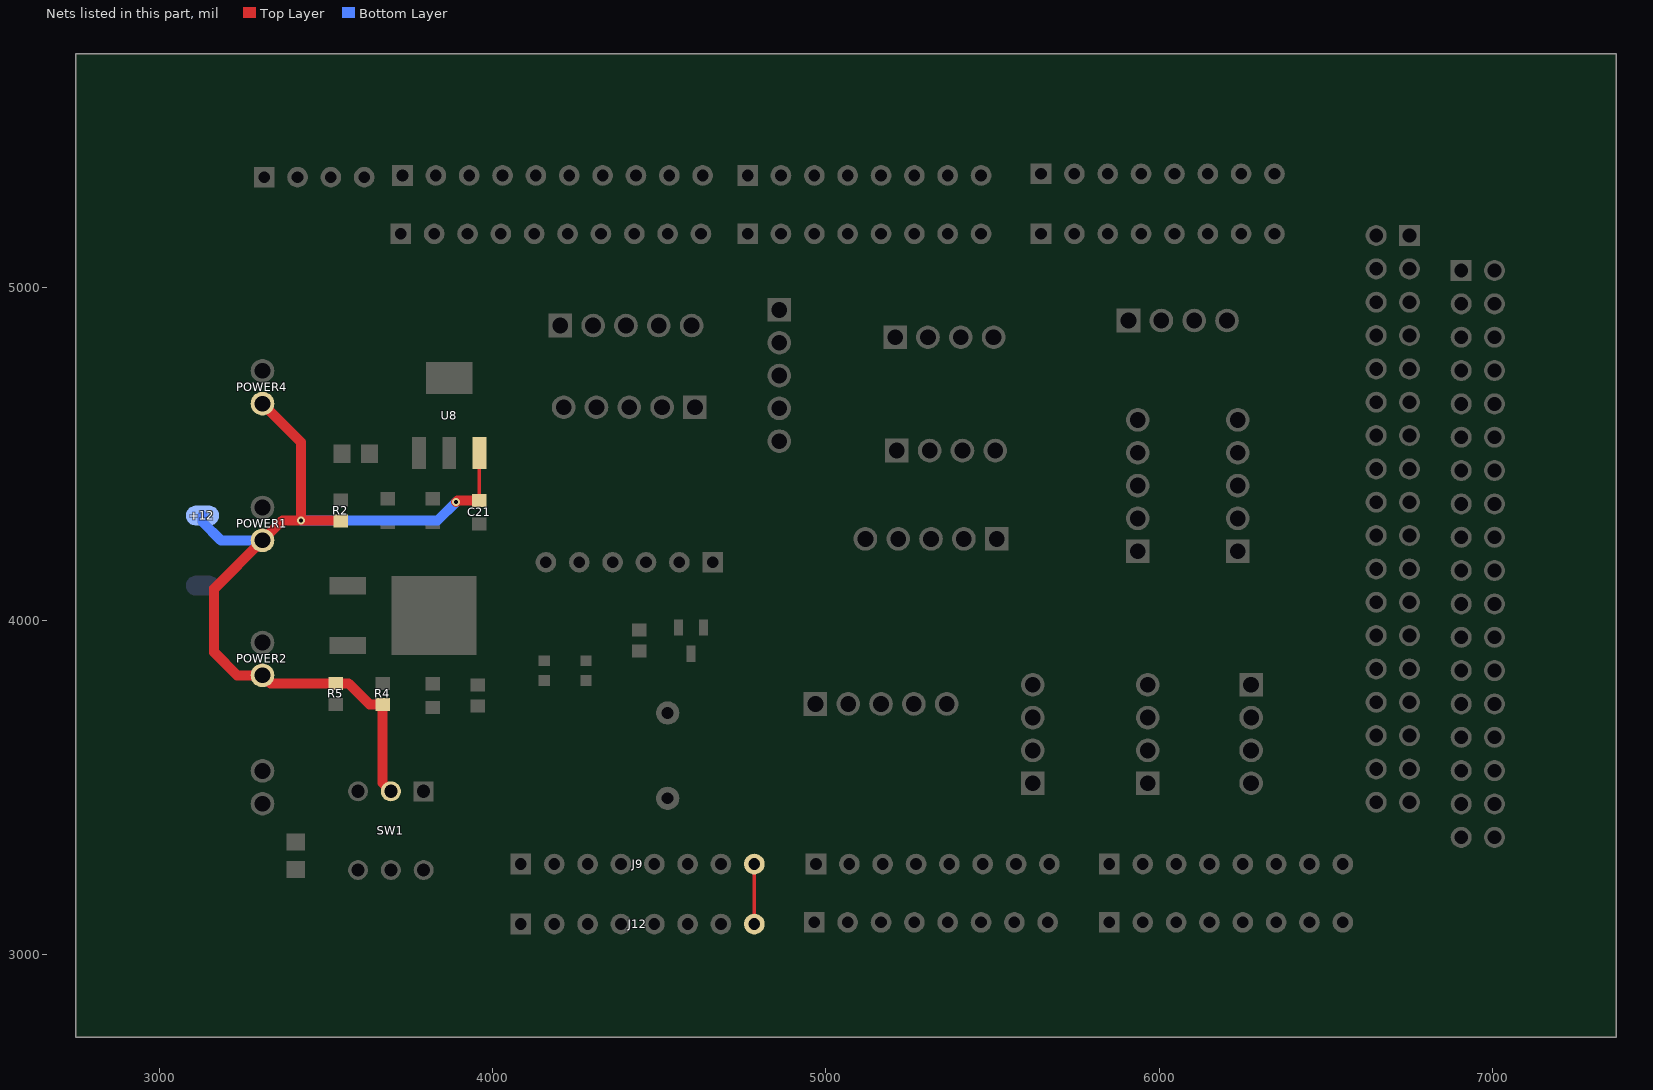
[diagram p0: the nets of this part, all layers, seen from the top]
# Altium PCB MISC49934.pcbdoc (part 2 of 2)
Units mil, origin at the board's own origin, x right, y up, seen from the top; angles counter-clockwise.
Board outline 4620 x 2950 mil, 2 copper layers (Top Layer, Bottom Layer), stack 0 mil thick; 53 components, 145 nets, 295 pads, 118 vias.

## Via types
v1: diameter 24, hole 12, Top Layer to Bottom Layer, 118 vias

## Nets (pads, with @x,y where several pads share a name; then routed paths per layer and width w, separated by ;. In a path a pad name is that pad's centre, name@x,y a point inside that pad or via, vN(x,y) a via of type N, cw(c..) or ccw(c..) an arc to the next point about the centre after c; other vN are vias at no path point) (continued)
VCC: +12.1 C21.2 POWER1.1 POWER2.1 POWER4.1 R2.2 R4.1 R5.1 SW1.2 U8.3 | length 2824.3
  Top Layer w10: C21.2@3960,4360.44 3960,4502 U8.3@3960.55,4502.5
  Top Layer w30: POWER2.1@3310,3835.7 3334.3,3811.5 R5.1@3530,3811.49 3568.5,3811.5 3631.5,3748.5 R4.1@3670,3748.51 3670,3513.1 SW1.2@3695.01,3488.11 ; POWER2.1@3310,3835.75 3234.25,3835.75 3165,3905 3165,4095.75 POWER1.1@3310,4240.75 3369.25,4300 v1(3425,4300) ; POWER4.1@3310,4650.7 3425,4535.7 v1(3425,4300) ; v1@3420,4300 v1(3425,4300) ; R2.2@3545,4298.5 3543.5,4300 v1(3425,4300) ; v1(3890,4355) 3895.4,4360.4 C21.2@3960,4360.44
  Bottom Layer w30: +12.1@3130,4315 3130,4295.7 3185,4240.7 POWER1.1@3310,4240.7 ; v1(3425,4300) 3835,4300 v1(3890,4355)
VIN: J9.8 J12.8 | length 180
  Top Layer w10: J12.8@4785,3090 J9.8@4785,3270
pads on no net: HC-06.1 HC-06.6 J9.1 J12.1 SW1.1 SW1.4 SW1.5 SW1.6 U8.4

## Polygon pours and split planes (outlines as drawn)
GND on Bottom Layer (solid, remove dead copper, pour order 4): 3005,5450 3000,5445 3000,3005 7110,3005 7110,5430
GND on Top Layer (solid, remove dead copper, pour order 4): 3000,5390 3005,5385 3005,3005 3010,3000 7120,3000 7105,3015 7105,5385

## Keep-outs
Board Outline Layer:
  lines w10: 3005.87,3173.07 ccw(c3025.55,3173.07) 3025.55,3153.39
  lines w10 net S$14301: 3005.87,3173.07 3005.87,5220.31 3006,5333 ; 3006,5324.53 cw(c3060,5330.87) 3065,5385
  lines w10 net S$3075: 6830.15,5240 6975,5240 7110,5105 7110,3285 6978.39,3153.39 6844.45,3153.39
  lines w10 net S$3947: 3890.47,3151 3907.3,3132.7 4030,3010 6610,3010 6705,3125 6729.9,3153.4
  lines w10 net S$3949: 3564,5385 3596,5385 3665,5385 6395,5385
  lines w10 net S$3952: 3055,5385 3519.55,5385
  lines w10 net S$3954: 6539.9,5240 6830.15,5240
  lines w10 net S$3958: 3025.55,3153.39 3887.66,3153.39
  lines w10 net S$3961: 3887.66,3153.39 3907.3,3133.75 3907.3,3132.7
  lines w10 net S$3963: 6705,3125 6729.9,3153.4
  lines w10 net S$3965: 6729.9,3153.39 6844.45,3153.39
  lines w10 net S$3975: 6395,5385 6539.9,5240
  lines w10 net S$3977: 3519.55,5385 3665,5385

## Other copper
Top Layer:
  drawing of 345 lines, arcs and shapes, not listed
Bottom Layer:
  region net OUT1_+5V: 3882.94,4411 3882.94,4429 3891.34,4425 3891.34,4415
  region net OUT1_+5V: 4172.06,4521 4172.06,4539 4163.66,4535 4163.66,4525
  region net VCC: 3150,4285 3110,4285 3163.79,4240.75 3195.61,4251.36
  region net VCC: 3286.56,4214.17 3286.56,4267.32 3261.76,4255.75 3261.76,4225.75
  region net +5V_3: 4697.94,4381 4697.94,4399 4706.34,4395 4706.34,4385
  region net +5V_3: 4902.06,4381 4902.06,4399 4893.66,4395 4893.66,4385
  region net D37: 6718.57,4353.03 6751.97,4386.43 6723.21,4388.86 6716.14,4381.79
  region net D37: 6326.98,4029.25 6314.25,4041.98 6323.02,4045.09 6330.09,4038.02
  region net D52: 6873.57,3448.03 6906.97,3481.43 6878.21,3483.86 6871.14,3476.79
  region net D52: 6679.02,3567.23 6658.51,3524.67 6686.32,3531.61 6690.92,3541.15
  region net D52: 6629.17,3531.38 6629.17,3578.62 6607.12,3560 6607.12,3550
  region net D52: 6556,3502.94 6574,3502.94 6570,3511.34 6560,3511.34
  region net D48: 5691.79,3347.26 5680.77,3333.02 5689.05,3330 5696.79,3340
  region net D48: 6646.76,3723.67 6619.32,3762.13 6612.15,3734.22 6618.04,3725.97
  region net D46: 6551,3952.06 6569,3952.06 6565,3945 6555,3945
  region net D46: 6618.57,3853.03 6651.97,3886.43 6623.21,3888.86 6616.14,3881.79
  region net D47: 6516,3977.06 6534,3977.06 6530,3968.66 6520,3968.66
  region net D47: 6536.14,3885.31 6519,3879.8 6520,3888.95 6530,3892.16
  region net D42: 6873.57,3948.03 6906.97,3981.43 6878.21,3983.86 6871.14,3976.79
  region net D42: 6679.02,4067.23 6658.51,4024.67 6686.32,4031.61 6690.92,4041.15
  region net D42: 6618.57,4056.97 6651.97,4023.57 6623.21,4021.14 6616.14,4028.21
  region net D42: 5261.19,3714.64 5298.79,3752.2 5301.06,3719.41 5293.99,3712.34
  region net D43: 5359.6,3714.64 5397.22,3752.19 5398.54,3720.33 5391.46,3713.27
  region net D43: 6718.57,4053.03 6751.97,4086.43 6723.21,4088.86 6716.14,4081.79
  region net D40: 6629.17,4131.38 6629.17,4178.62 6610,4160 6610,4150
  region net D40: 6541.98,4074.25 6529.25,4086.98 6538.02,4090.09 6545.09,4083.02
  region net D41: 6973.57,4048.03 7006.97,4081.43 6978.21,4083.86 6971.14,4076.79
  region net D41: 6770.83,4131.38 6770.83,4178.62 6792.88,4160 6792.88,4150
  region net D41: 6718.57,4153.03 6751.97,4186.43 6723.21,4188.86 6716.14,4181.79
  region net D41: 6541.98,4109.25 6529.25,4121.98 6538.02,4125.09 6545.09,4118.02
  region net D19: 6436,4957.94 6454,4957.94 6450,4966.34 6440,4966.34
  region net D19: 6174.8,5168.54 6132.8,5188.5 6158.32,5200.4 6167.91,5195.84
  region net D19: 6235.75,4733.02 6223.02,4745.75 6219.91,4736.98 6226.98,4729.91
  region net D39: 6973.57,4148.03 7006.97,4181.43 6978.21,4183.86 6971.14,4176.79
  region net D39: 6770.83,4231.38 6770.83,4278.62 6792.88,4260 6792.88,4250
  region net D39: 6744.14,4285.95 6720.03,4245.31 6710.49,4272.44 6715.75,4281.32
  region net D36: 6884.17,4226.38 6884.17,4273.62 6865,4255 6865,4245
  region net D36: 6679.02,4367.23 6658.51,4324.67 6686.32,4331.61 6690.92,4341.15
  region net D37: 6973.57,4248.03 7006.97,4281.43 6978.21,4283.86 6971.14,4276.79
  region net D37: 6770.83,4331.38 6770.83,4378.62 6792.88,4360 6792.88,4350
  region net D36: 6366.98,4029.25 6354.25,4041.98 6363.02,4045.09 6370.09,4038.02
  region net D28: 6873.57,4648.03 6906.97,4681.43 6878.21,4683.86 6871.14,4676.79
  region net D28: 6677.83,4769.76 6661.16,4725.55 6688.19,4734.74 6692.06,4745.01
  region net D35: 6748.03,4486.43 6781.43,4453.03 6783.86,4481.79 6776.79,4488.86
  region net D34: 6491.98,4334.25 6479.25,4346.98 6488.02,4350.09 6495.09,4343.02
  region net D34: 6629.17,4431.38 6629.17,4478.62 6607.12,4460 6607.12,4450
  region net D26: 6873.57,4748.03 6906.97,4781.43 6878.21,4783.86 6871.14,4776.79
  region net D26: 6648.03,4823.57 6681.43,4856.97 6683.86,4828.21 6676.79,4821.14
  region net D24: 6873.57,4848.03 6906.97,4881.43 6878.21,4883.86 6871.14,4876.79
  region net D24: 6648.03,4923.57 6681.43,4956.97 6683.86,4928.21 6676.79,4921.14
  region net D25: 6973.57,4848.03 7006.97,4881.43 6978.21,4883.86 6971.14,4876.79
  region net D25: 6770.83,4931.38 6770.83,4978.62 6792.88,4960 6792.88,4950
  region net D23: 6973.57,4948.03 7006.97,4981.43 6978.21,4983.86 6971.14,4976.79
  region net D23: 6770.83,5031.38 6770.83,5078.62 6792.88,5060 6792.88,5050
  region net D24: 6485.75,4838.02 6473.02,4850.75 6469.91,4841.98 6476.98,4834.91
  region net D24: 6391,4722.94 6409,4722.94 6405,4731.34 6395,4731.34
  region net +5V_1: 4183.06,3300.94 4215.94,3268.06 4218.38,3296.31 4211.31,3303.38
  region net +5V_1: 4501.85,3440.75 4501.85,3493.25 4477.35,3472 4477.35,3462
  region net D30: 6530.75,4143.02 6518.02,4155.75 6514.91,4146.98 6521.98,4139.91
  region net D30: 5500.31,3426.14 5494.8,3409 5503.95,3410 5507.16,3420
  region net D15: 4692.94,4346 4692.94,4364 4701.34,4360 4701.34,4350
  region net D51: 5816.98,3960.75 5804.25,3948.02 5811.46,3946.46 5818.54,3953.54
  region net D52: 5763.86,4019.69 5781,4025.2 5780,4016.05 5770,4012.84
  region net D52: 5766,3892.94 5784,3892.94 5780,3901.34 5770,3901.34
  region net D50: 5676.98,4075.75 5664.25,4063.02 5673.02,4059.91 5680.09,4066.98
  region net D50: 5726,3892.94 5744,3892.94 5740,3901.34 5730,3901.34
  region net D40: 5556.98,4094.25 5544.25,4106.98 5553.02,4110.09 5560.09,4103.02
  region net D41: 5547.94,4141 5547.94,4159 5556.34,4155 5556.34,4145
  region net +5V_4: 5462.94,4726 5462.94,4744 5471.34,4740 5471.34,4730
  region net +5V_4: 5585.75,4798.02 5573.02,4810.75 5569.91,4801.98 5576.98,4794.91
  region net D20: 5332.94,4701 5332.94,4719 5341.34,4715 5341.34,4705
  region net D20: 5600.49,4773.88 5594.53,4790.86 5587.75,4784.82 5591.42,4774.35
  region net D20: 6268.25,5139.5 6221.75,5139.5 6240,5117.8 6250,5117.8
  region net D20: 6196.98,4999.25 6184.25,5011.98 6193.02,5015.09 6200.09,5008.02
  region net D18: 6130.78,4923.44 6077.63,4923.44 6099.21,4948.24 6109.21,4948.24
  region net D18: 6043.06,5129.06 6075.94,5161.94 6078.38,5133.69 6071.31,5126.62
  region net D11: 4276.21,4637.78 4313.79,4675.36 4281,4677.65 4273.93,4670.57
  region net D1: 4309.73,5017.97 4291.81,5016.23 4296.58,5008.25 4306.58,5009.23
  region net D1: 4328.15,4908.43 4275,4908.44 4296.58,4933.24 4306.58,4933.24
  region net D11: 4339.72,5132.72 4296.09,5148.8 4305.23,5122.31 4315.57,5118.5
  region net D11: 4266.98,5064.25 4254.25,5076.98 4263.02,5080.09 4270.09,5073.02
  region net D8: 4116.14,4779.69 4099,4785.2 4100,4776.05 4110,4772.84
  region net D8: 4096,4707.94 4114,4707.94 4110,4716.34 4100,4716.34
  region net D15: 5001,4822.94 5019,4822.94 5015,4831.34 5005,4831.34
  region net D15: 5001,4887.06 5019,4887.06 5015,4878.66 5005,4878.66
  region net D49: 5831.98,4040.75 5819.25,4028.02 5828.02,4024.91 5835.09,4031.98
  region net D31: 6516,3697.94 6534,3697.94 6530,3706.34 6520,3706.34
  region net OUT1_+5V: 5080.75,4076.56 5068.02,4089.28 5064.91,4080.52 5071.98,4073.45
  region net OUT1_+5V: 4981.95,3976.09 4967.43,3986.72 4975.57,3991.17 4983.73,3985.19
  region net D7: 5885.75,3656.98 5873.02,3644.25 5869.91,3653.02 5876.98,3660.09
  region net D24: 6046,4562.94 6064,4562.94 6060,4571.34 6050,4571.34
  region net D24: 6046,4562.94 6064,4562.94 6060,4571.34 6050,4571.34
  region net D10: 4681,4992.06 4699,4992.06 4695,4983.66 4685,4983.66
  region net D10: 4824.64,4732.78 4862.22,4770.36 4829.42,4772.65 4822.35,4765.58
  region net D51: 5566,3967.94 5584,3967.94 5580,3976.34 5570,3976.34
  region net D51: 5563.86,4059.69 5581,4065.2 5580,4056.05 5570,4052.84
  region net D7: 5531.98,3980.75 5519.25,3968.02 5528.02,3964.91 5535.09,3971.98
  region net D7: 5697.06,3816 5697.06,3834 5688.66,3830 5688.66,3820
  region net D21: 5277.94,5016 5277.94,5034 5286.34,5030 5286.34,5020
  region net D15: 5410.75,4993.02 5398.02,5005.75 5396.46,4998.54 5403.54,4991.46
  region net D15: 5277.94,4986 5277.94,5004 5286.34,5000 5286.34,4990
  region net D14: 5527.06,5016 5527.06,5034 5518.66,5030 5518.66,5020
  region net D14: 5232.94,4956 5232.94,4974 5241.34,4970 5241.34,4960
  region net OUT1_+5V: 4824.64,4535.93 4862.22,4573.52 4829.43,4575.8 4822.35,4568.73
  region net OUT1_+5V: 4700.15,4571 4700.15,4589 4708.55,4585 4708.55,4575
  region net D7: 4770.75,5088.02 4758.02,5100.75 4754.91,5091.98 4761.98,5084.91
  region net D7: 4721,5007.94 4739,5007.94 4735,5016.34 4725,5016.34
  region net D39: 4407.78,4604.64 4445.36,4642.22 4447.65,4609.42 4440.58,4602.35
  region net OUT1_+5V: 5091.98,4087.78 5079.25,4100.51 5088.02,4103.62 5095.09,4096.55
  region net OUT1_+5V: 5144.72,4221.56 5091.57,4221.56 5113.15,4196.76 5123.15,4196.76
  region net D14: 5086,4837.94 5104,4837.94 5100,4846.34 5090,4846.34
  region net D14: 5086,4927.06 5104,4927.06 5100,4918.66 5090,4918.66
  region net D14: 5086,4927.06 5104,4927.06 5100,4918.66 5090,4918.66
  region net D20: 4831.53,4171.67 4821.86,4186.86 4831.03,4188.1 4836.53,4179.46
  region net D20: 4955.75,4293.02 4943.02,4305.75 4939.91,4296.98 4946.98,4289.91
  region net D14: 4935.75,4323.02 4923.02,4335.75 4919.91,4326.98 4926.98,4319.91
  region net D14: 4777.94,4201 4777.94,4219 4786.34,4215 4786.34,4205
  region net D48: 5060.75,4183.02 5048.02,4195.75 5044.91,4186.98 5051.98,4179.91
  region net D48: 4911.67,4056.53 4926.86,4046.86 4928.1,4056.03 4919.46,4061.53
  region net D2: 4966,4272.06 4984,4272.06 4980,4263.66 4970,4263.66
  region net D2: 4846.98,4114.25 4834.25,4126.98 4843.02,4130.09 4850.09,4123.02
  region net D31: 5655.16,3803.27 5611.26,3773.31 5642.99,3764.94 5651.4,3770.67
  region net D31: 5830.75,3596.98 5818.02,3584.25 5814.91,3593.02 5821.98,3600.09
  region net D31: 5840.31,3591.14 5834.8,3574 5843.95,3575 5847.16,3585
  region net D48: 4874.94,3397.01 4857.07,3394.85 4860,3403.67 4870,3404.87
  region net D48: 4856,3547.06 4874,3547.06 4870,3538.66 4860,3538.66
  region net D38: 5885.2,3486 5879.69,3468.86 5872.84,3475 5876.05,3485
  region net D38: 5461.98,3545.75 5449.25,3533.02 5458.02,3529.91 5465.09,3536.98
  region net D38: 4777.94,3586 4777.94,3604 4786.34,3600 4786.34,3590
  region net D38: 4907.06,3586 4907.06,3604 4898.66,3600 4898.66,3590
  region net OUT1_+5V: 5915.57,4572.22 5908.03,4624.83 5886.53,4600 5887.97,4590
  region net OUT1_+5V: 5667.06,4356 5667.06,4374 5658.66,4370 5658.66,4360
  region net OUT1_+5V: 5496.98,4380.75 5484.25,4368.02 5493.02,4364.91 5500.09,4371.98
  region net OUT1_+5V: 5496.98,4380.75 5484.25,4368.02 5493.02,4364.91 5500.09,4371.98
  region net D31: 6411,3872.94 6429,3872.94 6425,3881.34 6415,3881.34
  region net D31: 6510.75,4173.02 6498.02,4185.75 6494.91,4176.98 6501.98,4169.91
  region net D38: 6386,4022.06 6404,4022.06 6400,4013.66 6390,4013.66
  region net D38: 6386,3827.94 6404,3827.94 6400,3836.34 6390,3836.34
  region net D36: 6366.98,4030.75 6354.25,4018.02 6363.02,4014.91 6370.09,4021.98
  region net D36: 6361,3887.94 6379,3887.94 6375,3896.34 6365,3896.34
  region net D37: 6272.78,3547.71 6310.36,3510.13 6312.65,3542.93 6305.58,3550
  region net D37: 6306,4022.06 6324,4022.06 6320,4013.66 6310,4013.66
  region net D19: 6239.64,3608.57 6277.22,3646.15 6244.42,3648.44 6237.35,3641.37
  region net D19: 6174.8,5168.54 6132.8,5188.5 6158.32,5200.4 6167.91,5195.84
  region net D15: 5696,5067.94 5714,5067.94 5710,5076.34 5700,5076.34
  region net D15: 5714.06,5161.94 5746.94,5129.06 5718.69,5126.62 5711.62,5133.69
  region net D14: 5506,5107.06 5524,5107.06 5520,5098.66 5510,5098.66
  region net D14: 5535.75,5036.98 5523.02,5024.25 5519.91,5033.02 5526.98,5040.09
  region net +5V_3: 5332.37,4873.44 5279.22,4873.44 5300.79,4895.79 5310.79,4895.79
  region net +5V_3: 5702.06,4966 5702.06,4984 5693.66,4980 5693.66,4970
  region net D5: 4963.06,5190.94 4995.94,5158.06 4998.38,5186.31 4991.31,5193.38
  region net D5: 5894.85,4935.43 5919.85,4935.43 5912.35,4937.65 5902.35,4937.65
  region net D3: 5163.06,5190.94 5195.94,5158.06 5198.38,5186.31 5191.31,5193.38
  region net D3: 5988.44,3682.63 5988.44,3735.78 6013.24,3714.21 6013.24,3704.21
  region net D33: 5962.78,3843.01 6000.36,3805.43 6002.65,3838.22 5995.58,3845.3
  region net D6: 6262.5,3843.08 6287.5,3843.08 6280,3858.08 6270,3858.08
  region net D6: 6266,3952.06 6284,3952.06 6280,3943.66 6270,3943.66
  region net D2: 5265.75,5093.02 5253.02,5105.75 5249.91,5096.98 5256.98,5089.91
  region net D2: 5057.94,5016 5057.94,5034 5066.34,5030 5066.34,5020
  region net D2: 5041,5017.06 5059,5017.06 5055,5008.66 5045,5008.66
  region net D2: 5041,4682.94 5059,4682.94 5055,4691.34 5045,4691.34
  region net D6: 4863.06,5129.06 4895.94,5161.94 4898.38,5133.69 4891.31,5126.62
  region net D6: 5961,3967.94 5979,3967.94 5975,3976.34 5965,3976.34
  region net D33: 6565.75,4498.02 6553.02,4510.75 6549.91,4501.98 6556.98,4494.91
  region net D33: 6231.98,4034.25 6219.25,4046.98 6228.02,4050.09 6235.09,4043.02
  region net D34: 6003.57,4864.64 6041.15,4902.22 6043.44,4869.42 6036.37,4862.35
  region net D32: 6181,3882.94 6199,3882.94 6195,3891.34 6185,3891.34
  region net D32: 6560.75,4453.02 6548.02,4465.75 6544.91,4456.98 6551.98,4449.91
  region net D34: 6003.57,4864.64 6041.15,4902.22 6043.44,4869.42 6036.37,4862.35
  region net D34: 6351,4387.94 6369,4387.94 6365,4396.34 6355,4396.34
  region net D8: 4805.75,4071.98 4793.02,4059.25 4789.91,4068.02 4796.98,4075.09
  region net D8: 4377.94,4486 4377.94,4504 4386.34,4500 4386.34,4490
  region net D10: 4453.91,5171.2 4410.28,5187.28 4434.43,5201.5 4444.77,5197.69
  region net D10: 4681,5112.94 4699,5112.94 4695,5121.34 4685,5121.34
  region net D10: 4681,5097.06 4699,5097.06 4695,5088.66 4685,5088.66
  region net D10: 4681,5007.94 4699,5007.94 4695,5016.34 4685,5016.34
  region net Q2_3: 3336.57,3572.69 3283.43,3572.69 3305,3597.49 3315,3597.49
  region net _SDA: 3613.06,5299.06 3645.94,5331.94 3648.38,5303.69 3641.31,5296.62
  region net _SDA: 3844.72,5307.72 3801.09,5323.8 3810.23,5297.31 3820.57,5293.5

## Silkscreen, mask and mechanical layers (free items; w line width, h text height)
Top Silkscreen Layer:
  lines w10 net S$11567: 3355.56,5195 3355.56,5280 ; 3465.56,5195 3465.56,5280 ; 3660,5192.5 3660,5277.5 ; 4235,4410 4235,4502.2 ; 4295,4225 4295,4315 ; 4339.28,4410 4339.28,4502.2 ; 4405,4225 4405,4320 ; 4453,4502.2 4453.28,4410 ; 4504,4225 4505,4325 ; 4559,4502.2 4560,4410 ; 4605,4320 4605.5,4225 ; 4665,4410 4665,4502.2 ; 5005,3565 5005,3659.45 ; 5109.01,3659.45 5110,3570 ; 5200,3570 5201.01,3659.45 ; 5298.01,3574.45 5298.01,3659.45 ; 5405.01,3574.45 5405.01,3659.45 ; 5715,3680 5800,3680 ; 5716,3482.39 5801,3482.39 ; 5716,3574.39 5801,3574.39 ; 5716,3784.39 5801,3784.39 ; 6061,3476.97 6146,3476.97 ; 6061,3579.36 6146,3579.36 ; 6061,3673.86 6146,3673.86 ; 6061,3778.91 6146,3778.91 ; 6408,3484.74 6493,3484.74 ; 6408,3585.46 6493,3585.46 ; 6408,3695.75 6493,3695.75 ; 6408,3786.86 6493,3786.86
  lines w10 net S$11623: 3560,5190 3560,5277.44 3562.56,5280
  lines w10 net S$12201: 5345,4650 5345,4720
  lines w10 net S$12203: 5445,4650 5445,4720
  lines w10 net S$12205: 5558.54,4643 5558.54,4715
  lines w10 net S$12209: 5230.82,4643 5230.82,4720
  lines w10 net S$12241: 5225.7,4983 5225.7,5050
  lines w10 net S$12243: 5329.7,4983 5329.7,5050
  lines w10 net S$12245: 5433.7,4983 5433.7,5055
  lines w10 net S$12247: 5539.7,4983 5539.7,5055
  lines w10 net S$12361: 6325,4176.58 6410,4176.58
  lines w10 net S$12363: 6325.55,4277.78 6390,4277.78
  lines w10 net S$12365: 6325.55,4393.78 6400,4393.78
  lines w10 net S$12369: 6325,4586.78 6405,4586.78
  lines w10 net S$12371: 6325.55,4490.28 6405,4490.28
  lines w10 net S$12373: 5932.39,4745 5932.39,4804
  lines w10 net S$12375: 6034.39,4804 6035,4745
  lines w10 net S$12377: 6135.39,4740 6135.39,4804
  lines w10 net S$12379: 6245,4740 6245,4804
  lines w10 net S$12417: 4997.8,4914.7 5080,4914.7
  lines w10 net S$12419: 4997.8,4798.27 5080,4798.27
  lines w10 net S$12421: 4997.8,4720.41 5080,4720.41
  lines w10 net S$12423: 4997.8,4607.56 5080,4607.56
  lines w10 net S$12425: 4997.8,4501.41 5065,4501.41
  lines w10 net S$12427: 5065,4501.41 5080,4501.41
  lines w10 net S$12429: 4231.58,4745 4231.58,4795
  lines w10 net S$12431: 4336.27,4745 4336.27,4794.45
  lines w10 net S$12433: 4454.41,4745 4454.41,4794.45
  lines w10 net S$12435: 4570,4745 4570,4795
  lines w10 net S$12437: 4682.53,4745 4682.53,4794.45
  lines w10 net S$12583: 5155.87,4015 5155.87,4107.2
  lines w10 net S$12586: 5262.53,4015 5262.53,4107.2
  lines w10 net S$12588: 5355.37,4015 5355.37,4107.2
  lines w10 net S$12590: 5458.87,4015 5458.87,4107.2
  lines w10 net S$12592: 5580.87,4015 5580.87,4107.2
  lines w10 net S$12594: 5710,4572.15 5797.2,4572.15
  lines w10 net S$12596: 5705,4464.15 5797.2,4464.15
  lines w10 net S$12598: 5705,4348.15 5797.2,4348.15
  lines w10 net S$12601: 5700,4268.15 5797.2,4268.15
  lines w10 net S$12603: 5700,4155.81 5797.2,4155.81
  lines w10 net S$14520: 3330,4850 3405,4775 3405,4360
  lines w10 net S$3942: 3310,3740 3330,3740 3405,3815 3405,4360
  text "D6" at 4855,5240 h39.37
  text "D15" at 5730,5240 h39.37
  text "D21" at 6330,5239.6 h39.37
  text "AREF" at 3895,5235 h39.37
  text "GND" at 4010,5235 h39.37
  text "D12" at 4205,5235 h39.37
  text "D11" at 4310,5235 h39.37
  text "D10" at 4410,5235 h39.37
  text "D9" at 4510,5235 h39.37
  text "D8" at 4615,5235 h39.37
  text "D7" at 4750,5234.6 h39.37
  text "D5" at 4950,5235 h39.37
  text "D4" at 5050,5234.6 h39.37
  text "D3" at 5160,5235 h39.37
  text "D2" at 5250,5234.6 h39.37
  text "D1" at 5355,5234.6 h39.37
  text "D0" at 5450,5235 h39.37
  text "D14" at 5625,5234.6 h39.37
  text "D16" at 5825,5235 h39.37
  text "D17" at 5920,5234.6 h39.37
  text "D18" at 6030,5235 h39.37
  text "D19" at 6130,5235.2 h39.37
  text "D20" at 6230,5235 h39.37
  text "SCL" at 3700,5230 h39.37
  text "SDA" at 3805,5230 h39.37
  text "D13" at 4105,5230 h39.37
  text "SCL" at 3440,5185 h59.05 r90
  text "+5V" at 3535,5185 h59.05 r90
  text "SDA" at 3340,5170 h59.05 r90
  text "GND" at 3635,5165 h59.05 r90
  text "5V" at 6540,5145 h39.37
  text "5V" at 6810,5145 h39.37
  text "D23" at 6810,5110 h39.37 r270
  text "TX" at 5670,5065 h59.05 r90
  text "TX" at 5870,5065 h59.05 r90
  text "RX" at 5770,5060 h59.05 r90
  text "RX" at 5965,5055 h59.05 r90
  text "Servo signal line" at 4370,5050 h59.05
  text "RX" at 6070,5050 h59.05 r90
  text "TX" at 6165,5050 h59.05 r90
  text "D22" at 6535,5035 h39.37
  text "SDA" at 6265,5030 h59.05 r90
  text "SCL" at 6370,5030 h59.05 r90
  text "V0.2" at 3255,4995 h59.05
  text "GND" at 5220,4990 h43.31 r90
  text "D49" at 5420,4990 h43.31 r90
  text "D50" at 5525,4990 h43.31 r90
  text "+5V" at 5325,4985 h43.31 r90
  text "D25" at 6815,4985 h39.37 r270
  text "D24" at 6535,4945 h39.37
  text "GND" at 5010,4925 h43.31
  text "D26" at 6815,4885 h39.37 r270
  text "D26" at 6540,4835 h39.37
  text "OUT" at 5015,4820 h43.31
  text "PWC" at 5890,4795 h43.31 r270
  text "IN3" at 5975,4795 h43.31 r270
  text "A3" at 6080,4790 h43.31 r270
  text "B3" at 6180,4790 h43.31 r270
  text "D29" at 6815,4770 h39.37 r270
  text "Output" at 3060,4745 h78.74
  text "S3" at 4370,4745 h59.05
  text "S4" at 4490,4745 h59.05
  text "S5" at 4600,4745 h59.05
  text "S1" at 4160,4740 h59.05
  text "S2" at 4255,4740 h59.05
  text "D29" at 6535,4735 h39.37
  text "S2" at 5015,4730 h43.31
  text "D31" at 6815,4680 h39.37 r270
  text "+5V" at 5330,4660 h59.05 r90
  text "D51" at 5425,4655 h59.05 r90
  text "GND" at 5225,4650 h43.31 r90
  text "D52" at 5545,4650 h59.05 r90
  text "D30" at 6540,4635 h39.37
  text "Power" at 3060,4630 h78.74
  text "S3" at 5020,4625 h43.31
  text "+5V" at 5720,4595 h43.31
  text "+5V" at 6330,4590 h43.31
  text "D33" at 6815,4580 h39.37 r270
  text "D32" at 6540,4540 h39.37
  text "+5V" at 5005,4505 h43.31
  text "L" at 6355,4500 h43.31
  text "L" at 5735,4490 h43.31
  text "D35" at 6810,4475 h39.37 r270
  text "S1" at 4165,4435 h59.05
  text "LED" at 4350,4435 h59.05
  text "S0" at 4260,4430 h59.05
  text "D34" at 6535,4430 h39.37
  text "C" at 6345,4410 h43.31
  text "+5V" at 4630,4400 h59.05 r90
  text "C" at 5735,4395 h43.31
  text "GND" at 4530,4385 h59.05 r90
  text "D37" at 6810,4385 h39.37 r270
  text "D36" at 6535,4345 h39.37
  text "Servo" at 3050,4330 h78.74
  text "R" at 6350,4290 h43.31
  text "R" at 5740,4280 h43.31
  text "D39" at 6815,4280 h39.37 r270
  text "Bluetooth" at 4075,4260 h59.05
  text "RX" at 4480,4250 h59.05 r90
  text "TX" at 4580,4250 h59.05 r90
  text "D38" at 6540,4240 h39.37
  text "+5V" at 4280,4235 h59.05 r90
  text "GND" at 4380,4235 h59.05 r90
  text "Power" at 3045,4230 h78.74
  text "GND" at 6330,4190 h43.31
  text "GND" at 5700,4185 h43.31
  text "D41" at 6815,4175 h39.37 r270
  text "D40" at 6540,4145 h39.37
  text "+5V" at 5090,4100 h59.05 r270
  text "GND" at 5490,4100 h59.05 r270
  text "LED" at 5195,4090 h59.05 r270
  text "D43" at 6820,4075 h39.37 r270
  text "D42" at 6535,4045 h39.37
  text "S0" at 5290,4035 h59.05
  text "S1" at 5385,4035 h59.05
  text "D45" at 6820,3980 h39.37 r270
  text "D44" at 6535,3920 h39.37
  text "Motor" at 3045,3915 h78.74
  text "OUT-12V" at 3485,3895 h59.05 r90
  text "D47" at 6815,3885 h39.37 r270
  text "D46" at 6535,3835 h39.37
  text "Power" at 3045,3825 h78.74
  text "B2" at 6070,3795 h59.05
  text "PWD" at 6420,3795 h59.05
  text "B1" at 5725,3790 h59.05
  text "D49" at 6815,3775 h39.37 r270
  text "D48" at 6535,3740 h39.37
  text "IN4" at 6420,3700 h59.05
  text "A2" at 6065,3695 h59.05
  text "A1" at 5725,3690 h59.05
  text "D51" at 6815,3675 h39.37 r270
  text "D50" at 6540,3645 h39.37
  text "S3" at 5330,3595 h59.05
  text "S2" at 5230,3590 h59.05
  text "IN2" at 6065,3590 h59.05
  text "A4" at 6420,3590 h59.05
  text "IN1" at 5725,3585 h59.05
  text "D53" at 6820,3575 h39.37 r270
  text "+5V" at 4985,3560 h59.05 r90
  text "OUT" at 5180,3550 h59.05 r90
  text "GND" at 5090,3545 h59.05 r90
  text "D52" at 6540,3545 h39.37
  text "Input" at 3060,3540 h78.74
  text "PWA" at 5720,3495 h59.05
  text "PWB" at 6065,3495 h59.05
  text "B4" at 6420,3495 h59.05
  text "Power" at 3060,3440 h78.74
  text "IN12V" at 3430,3425 h59.05 r90
  text "GND" at 6605,3370 h39.37
  text "GND" at 6715,3370 h39.37
  text "RESEF" at 4300,3310 h31.5 r90
  text "A8" at 5825,3170 h31.5
  text "A0" at 4940,3165 h31.5
  text "A1" at 5045,3165 h31.5
  text "A2" at 5150,3165 h31.5
  text "A3" at 5240,3165 h31.5
  text "A4" at 5345,3165 h31.5
  text "A5" at 5440,3165 h31.5
  text "A6" at 5540,3165 h31.5
  text "A7" at 5645,3165 h31.5
  text "A9" at 5925,3165 h31.5
  text "A10" at 6015,3165 h31.5
  text "A11" at 6115,3165 h31.5
  text "A12" at 6215,3165 h31.5
  text "A13" at 6315,3165 h31.5
  text "A14" at 6415,3165 h31.5
  text "A15" at 6520,3165 h31.5
  text "5V" at 4165,3160 h31.5
  text "3.3V" at 4335,3160 h31.5
  text "5V" at 4455,3160 h31.5
  text "GND" at 4545,3160 h31.5
  text "GND" at 4640,3160 h31.5
  text "VIN" at 4750,3160 h31.5
Bottom Silkscreen Layer:
  text "Arduino-2560 expansion board" at 3960,4195 h59.05
  text "V0.2" at 3485,4130 h59.05

## Dimensions
4675.35,5320.86 to 4714.72,5320.86 on Document Layer
5515,5280 to 5593.74,5280 on Document Layer
6396.6,5266.64 to 6593.45,5266.64 on Document Layer
6665,3400 to 6665,3321.26 on Document Layer
4914.4,3207.03 to 4835.66,3207.03 on Document Layer
4035,3077.99 to 3005,3077.99 on Document Layer
5720.35,3197.06 to 5799.09,3197.06 on Document Layer
4147.92,3215.12 to 4147.92,5104.88 on Document Layer
5739.65,3315.12 to 5739.65,5204.88 on Document Layer